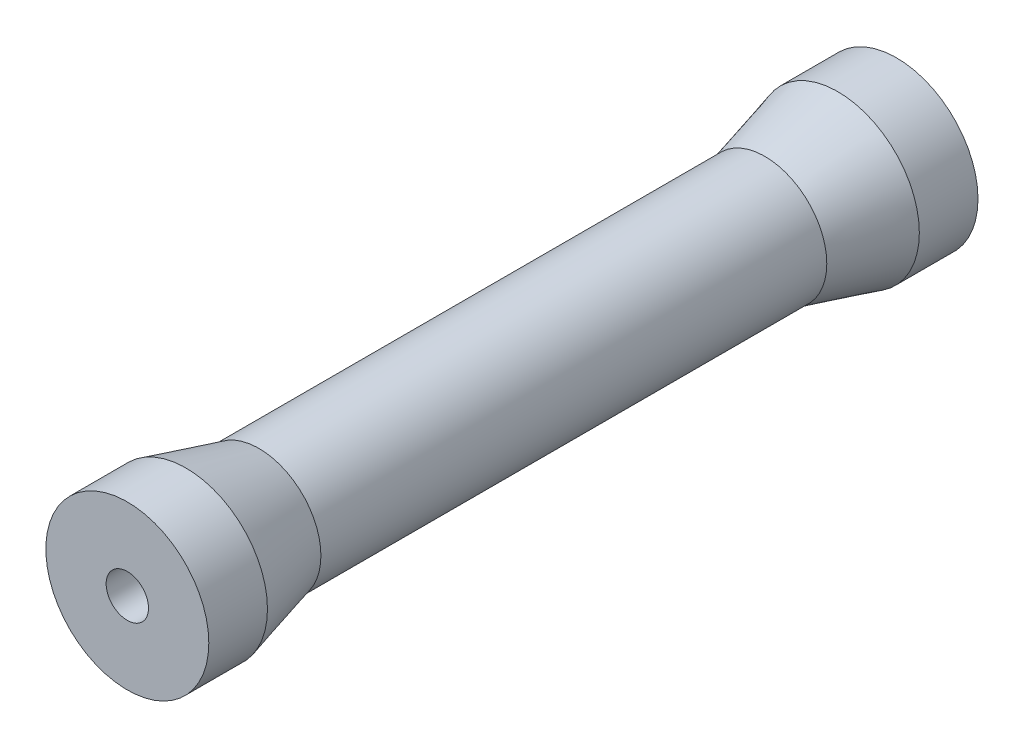
SolidWorks part; units mm, degrees
ref_plane "Front" through (0, 0, 0) normal (0, 0, 1) x (1, 0, 0)
ref_plane "Top" through (0, 0, 0) normal (0, 1, 0) x (1, 0, 0)
ref_plane "Right" through (0, 0, 0) normal (1, 0, 0) x (0, 0, -1)
sketch "Sketch1" plane through (0, 0, 0) normal (0, 0, 1) x (1, 0, 0)
  circle A0 centre (0, 0) radius 3.25
  circle A1 centre (0, 0) radius 12.5
  dimension "D1" = 6.5
  dimension "D2" = 25
extrude "Boss-Extrude1" add sketch "Sketch1" along normal mid plane 118
sketch "Sketch3" plane through (0, 0, 0) normal (0, 1, 0) x (1, 0, 0)
  line L0 (12.5, -50) -> (12.5, 50)
  line L1 (12.5, 50) -> (9.5, 38.8038)
  line L2 (9.5, 38.8038) -> (9.5, -38.8038)
  line L3 (9.5, -38.8038) -> (12.5, -50)
  line L4 (0, 0) -> (20.1418, 0) construction
  line L5 (12.5, -59) -> (12.5, 59) construction
  line L6 (0, 0) -> (0, 62.3065) construction
  dimension "D1" = 15
  dimension "D2" = 15
  dimension "D3" = 3
  dimension "D4" = 100
revolve "Cut-Revolve1" cut sketch "Sketch3" angle 360 about L6
